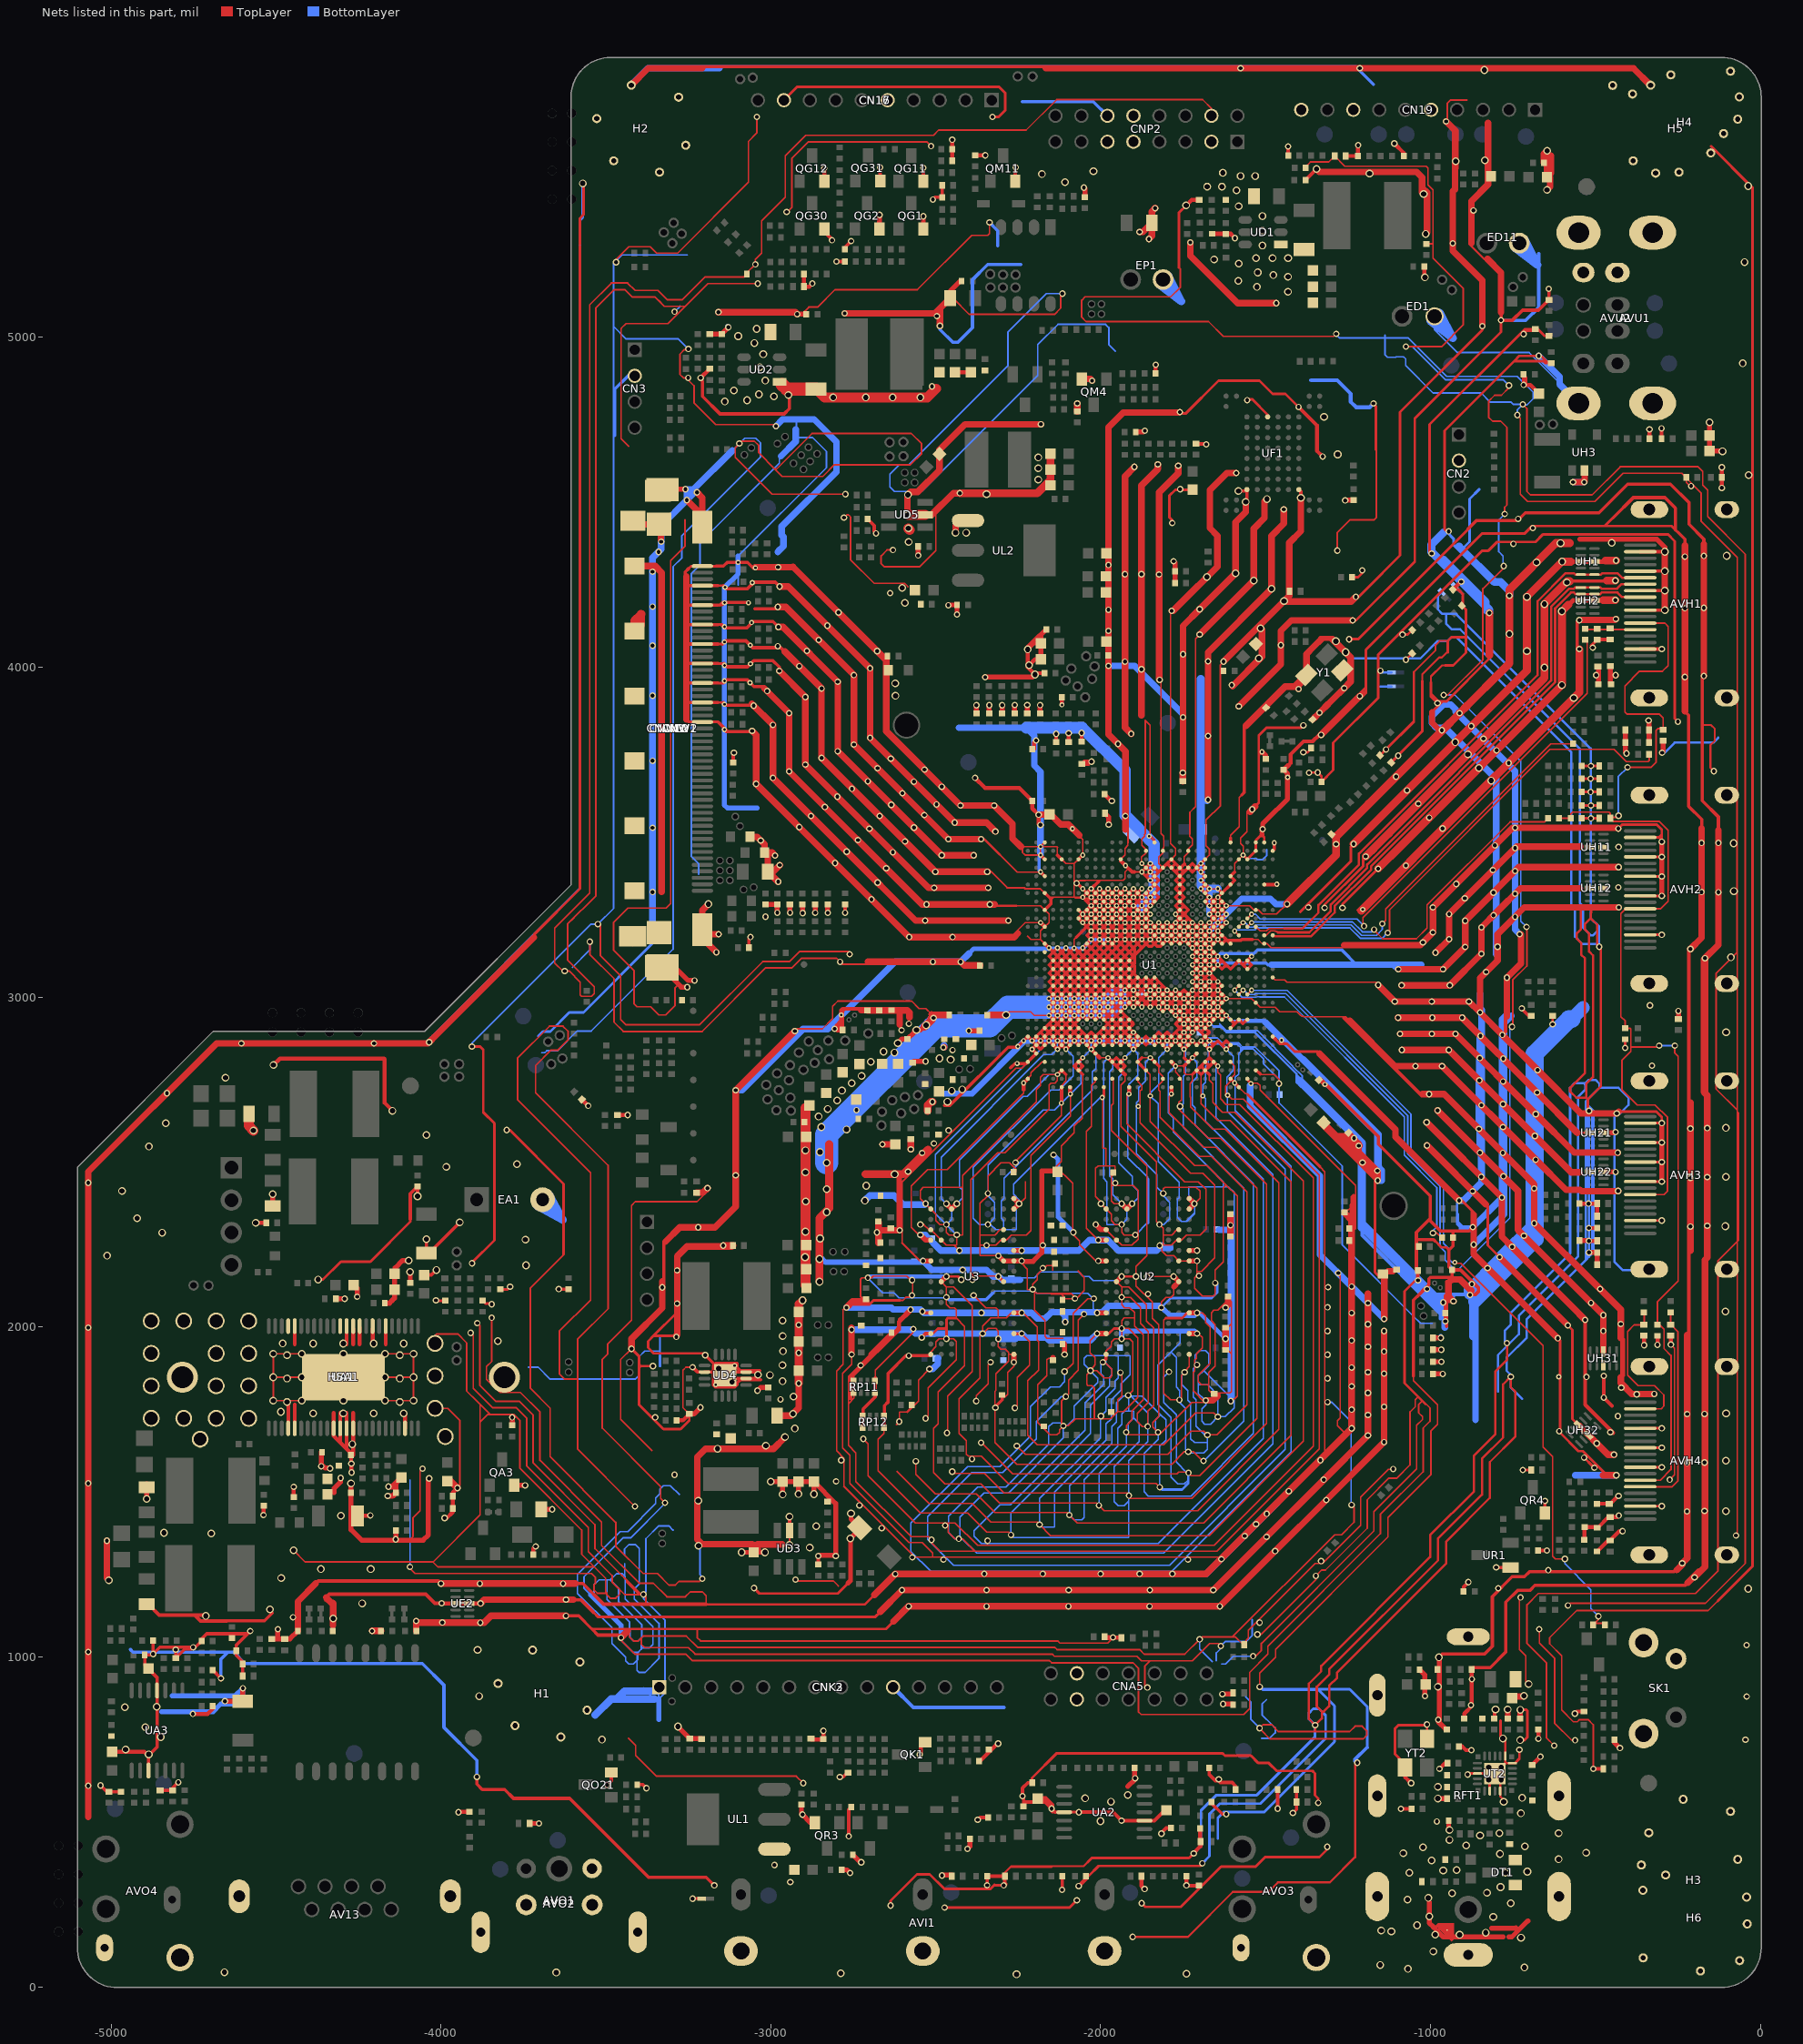
[diagram p0: the nets of this part, all layers, seen from the top]
# Altium PCB MISC86290.PcbDoc (part 21 of 31)
Units mil, origin at the board's own origin, x right, y up, seen from the top; angles counter-clockwise.
Board outline 5104.71 x 5851.49 mil, 2 copper layers (TopLayer, BottomLayer), stack 61.855 mil thick; 1026 components, 667 nets, 4280 pads, 2294 vias.

## Via types
v1: diameter 19.68, hole 11.81, TopLayer to BottomLayer, tented both sides, 1189 vias
v2: diameter 19.68/19.68 (per signal layer), hole 11.81, TopLayer to BottomLayer, tented both sides, 366 vias
v3: diameter 15.75, hole 7.87, TopLayer to BottomLayer, tented both sides, 348 vias
v4: diameter 23.62, hole 15.75, TopLayer to BottomLayer, tented both sides, 309 vias
v5: diameter 15.75/15.75 (per signal layer), hole 7.87, TopLayer to BottomLayer, tented both sides, 59 vias
v6: diameter 24/24 (per signal layer), hole 16, TopLayer to BottomLayer, tented both sides, 23 vias

## Nets (pads, with @x,y where several pads share a name; then routed paths per layer and width w, separated by ;. In a path a pad name is that pad's centre, name@x,y a point inside that pad or via, vN(x,y) a via of type N, cw(c..) or ccw(c..) an arc to the next point about the centre after c; other vN are vias at no path point) (continued)
GND: (continued)
  BottomLayer w15.75: v6@-2849.72,2268.03 -2849.72,2212.2 -2833.98,2196.46 -2542.64,2196.46 v2(-2538.7,2200.39) ; v2(-1936.34,1964.17) -1936.34,1991.73 -1932.4,1987.8 -1759.17,1987.8 -1715.87,1987.8 v2(-1707.99,1979.92) ; v3@-1925.81,2867.72 v3(-1900.91,2867.72) v3@-1867.72,2867.72 ; v3@-1920.59,2867.72 -1910.75,2857.87 ; -1889.09,2857.87 -1879.25,2867.72 v3@-1867.72,2867.72 ; -1857.6,2865.75 -1857.6,2867.72 v3@-1867.72,2867.72 ; v2(-1816.26,2058.66) -1814.29,2058.66 -1790.67,2035.04 -1715.87,2035.04 v2(-1707.99,2042.91)
  BottomLayer w18: -2471.72,2708.03 -2389.72,2708.03 -2230.04,2867.72 -2117.44,2867.72 v3@-1920.59,2867.72
  BottomLayer w19.68: v2(-2770.98,2058.66) -2635.16,2058.66 -2629.25,2052.76 v2(-2576.1,2052.76) -2546.57,2052.76 v2(-2540.67,2046.85) -2536.73,2042.91 v2(-2361.54,2042.91) v2(-2239.49,2042.91) -2209.96,2042.91 -2192.24,2025.2 -2168.62,2025.2 -2148.94,2044.88 -2119.41,2044.88 ; v2(-2755.24,1991.73) -2574.13,1991.73 -2562.32,1979.92 v2(-2357.6,1979.92) v2(-2239.49,1979.92) v2@-2237.66,1978.09 ; v2@-2547.82,2279.13 -2532.07,2279.13 -2484.83,2231.89 ; v2(-2546.57,2279.13) -2530.83,2279.13 ; v2(-2538.7,2200.39) -2511.14,2172.83 v2(-2418.62,2172.83) -2345.79,2172.83 -2326.1,2153.15 v2(-2310.35,2153.15) ; -2483.58,2231.89 v2(-2428.46,2231.89) v2(-2239.49,2231.89) -2066.26,2231.89 -2034.76,2263.39 -1977.68,2263.39 -1946.18,2231.89 -1830.04,2231.89 v2@-1822.25,2239.68 ; v2@-2237.6,1978.03 -2227.68,1968.11 -2164.88,1968.11 -2157.01,1960.24 -2030.83,1960.24 v2(-2011.14,1979.92) ; v2(-2107.6,2015.35) -2107.6,2033.07 -2119.41,2044.88 ; -1897.31,4004.31 v1@-1750.25,3857.25 ; v2(-1816.26,2058.66) -1822.17,2064.57 -1975.71,2064.57 -1995.39,2044.88 -2119.41,2044.88 ; v2@-1814.29,2247.64 v2@-1822.25,2239.68 ; C95.1@-1788.7,2239.59 -1822.17,2239.59 v2@-1822.25,2239.68 ; v1@-1678.07,3594.68 v1(-1674.72,3598.03) ; v3(-1670.59,3200.39) -1572.48,3298.5 -1485.5,3298.5 -1469.21,3282.21 v1(-1434.96,3282.21) ; C85.1@-1640.75,2294.88 -1611.54,2294.88 -1605.63,2288.98 -1605.63,1785.92 v2(-1605.63,1775.2) ; -1501.73,2924.84 -1454.45,2877.56 -1436.82,2859.93
  BottomLayer w20: v4(-3570.25,5467) v4@-3569.83,5466.58 ; H2.3@-3424.48,5764.76 -3373.28,5815.96 -3156.25,5815.96 ; -3358.61,3183 -3358.61,3267 ; -3358.61,3223.74 -3358.61,3267 ; -3332.25,4428.59 -3332.25,4428.75 ; v1@-3224.72,4531.02 -3229.98,4531.02 v1@-3251.75,4509.25 ; -3116.5,4657.2 -3235.31,4538.38 -3254,4538.38 -3254,4511.5 v1@-3251.75,4509.25 ; v1@-3106,2718.25 -3086.97,2718.25 -2902.21,2903 -2827.32,2903 -2623.32,3107 v1(-2509,3107) v1(-2424.51,3107) -2399.15,3132.36 ; v1(-2984.5,4731) -2964.16,4751.34 -2868.71,4751.34 ; -2979,4350 -2976.94,4352.06 -2976.53,4352.06 -2961.97,4366.61 -2961.97,4394.97 -2967,4400 -2967,4426.66 -2801,4592.66 -2801,4683.63 -2868.71,4751.34 ; -2969,4639.91 -2924.41,4684.5 -2924.41,4720.59 ; -2893.66,4751.34 -2868.71,4751.34 ; v6@-2715.97,2383.03 -2700.28,2398.72 ; v6(-2714.72,2383.03) -2699.03,2398.72 -2626.42,2398.72 -2598.42,2370.72 -2533.72,2370.72 v2(-2530.83,2373.62) ; v2(-2519.02,1872.64) -2509.72,1872.64 -2493.72,1888.64 -2493.72,1904.5 C94.1@-2493.11,1905.12 ; v1@-2475,2848 v1@-2475,2854.32 ; -2430,3817 -2225.58,3817 -2201.16,3792.58 -2201.16,3702.01 -2182.4,3683.26 v3(-2182.4,3430.71) ; v2(-2310.35,1964.17) -2257.72,1964.17 -2253.79,1968.11 -2227.68,1968.11 ; v2@-2304.76,2149.21 -2298.54,2142.99 -2290.72,2142.99 ; C93.1@-2270.98,2142.99 -2290.72,2142.99 ; -2243.72,2142.99 -2290.72,2142.99 ; v1(-1976.45,4004.31) -1926,4004.31 ; v1(-1926.45,4017) -1926,4016.55 -1926,4004.31 ; v3(-1900.91,2867.72) -1845.79,2867.72 -1843.82,2865.75 -1857.6,2865.75 ; -1897.31,4004.31 -1926,4004.31 ; -1680.29,1251.34 v2(-1529,1402.63) -1465.58,1466.06 ; v3@-1670.59,3252.21 v3(-1670.59,3328.35) ; v3@-1546.69,2733 -1546.69,2670.24 -1335.17,2458.73 -1335.17,2218.44 v1(-1239.22,2122.5) v1(-1140.72,2024) ; -1481.85,3098.03 -1122,3098.03 ; -1454.45,2877.56 -1425.67,2848.78 -1357.44,2780.56 ; -1384.92,2811.31 -1157.91,2584.3 -1157.91,2476.95 v1(-1161.28,2473.58) ; -1309.76,2732.87 -1357.44,2780.56 ; -1203.17,2307.5 -1203.17,2295.67 -970.5,2063 ; -1182.77,2607.6 -1220.09,2644.91 ; v1@-1161.73,2474.02 -1161.73,2586.55 -1220.09,2644.91 ; v1@-1160.5,2474.36 v1(-1160.5,2444) -1148.5,2444 -1147.5,2445 -1147.5,2475.02 -1159.01,2486.54 -1159.01,2509 ; v1(-1097.72,3084.85) -1110.9,3098.03 -1122,3098.03 ; -1028.32,3098.03 -1122,3098.03 ; -970.5,2081.5 -961.5,2072.5 -957,2072.5 -957,2091.5 -935.76,2091.5 ; -957,1999 -957,2054 ; v1@-913.5,2383.45 -900.55,2383.45 v1(-872.4,2411.6) -844.84,2439.16 v1@-844.84,2453.55 ; -905.29,2298.16 -876.84,2298.16 v1(-872,2303) v1@-783,2392 ; v1(-869.43,2249.54) -783,2336 ; -864,1719 -864,1962 ; -850.23,3010.77 -850.23,2966.38 -844.84,2961 v1@-844.84,2453.55 ; v1(-848.42,2882.42) -850.57,2880.28 v1(-850.57,2815.28) -852.21,2813.63 v1(-852.21,2747.63) -853.27,2746.57 -853.27,2664.57 ; -846.29,2470 v1@-846.29,2456.21 ; v1(-845.86,2671.98) -853.27,2664.57 ; v1(-811,3385) -800.84,3395.16 -800.84,3398 ; v1(-809.31,3317.06) -800.84,3325.53 -800.84,3331 ; v1(-804.9,3460.06) -800.84,3456 -800.84,3419 ; -800.84,3130.84 -800.84,3331 ; v1@-783,2885.54 -783,2854.5 ; -772.84,2943 -783,2932.84 -783,2854.5 ; -754.63,2943.5 -777.84,2920.29 -777.84,2394.66 -777.18,2394 -777.18,2341.82 -783,2336 ; -747,2181.13 -792.5,2135.63 ; v1(-730,3191) -743.84,3204.84 -743.84,3685.26 -923.79,3865.21 -923.79,3871.92 -938.71,3886.84 -960.29,3886.84 -995.84,3851.29 -995.84,3830.71 -981.29,3816.16 -960.71,3816.16 -958.03,3818.84 -800.84,3661.65 -800.84,3419 ; -677.5,2331.26 -692.18,2316.57 -792.5,2216.26 -792.5,2199.5 -792.5,2161.5 ; v1(-672,4944) -609,4881 -609,4862 -609,4858.21 AVU2.9@-551.16,4800.38 ; v1(-568,4561.43) v1(-534,4561.43) ; -561,1550.66 v2(-437,1550.66) ; -3358.61,3267 -3358.61,4331.67 -3332.41,4357.88 v1(-3332.41,4380.97) -3332.41,4428.59 -3332.25,4428.75 ; -3332.25,4428.75 v1@-3251.75,4509.25 ; -1357.44,2780.56 -1355.73,2780.56 -1220.09,2644.91 ; -864,1962 -864,2064.13 -792.5,2135.63 ; -864,1962 -873,1971 -873,2081 -792.5,2161.5 ; -853.27,2664.57 v1(-853.27,2600.57) -850.42,2597.72 v1(-850.42,2528.42) -846.29,2524.3 v1@-846.29,2456.21 ; v1@-846.29,2456.21 v1(-846.29,2455) v1@-844.84,2453.55 ; -800.84,3331 -800.84,3398 ; -800.84,3398 -800.84,3419 ; -792.5,2135.63 -792.5,2149.77 -792.5,2161.5 ; -783,2336 v1@-783,2392 ; v1@-783,2392 -783,2854.5
  BottomLayer w23: -3532.25,824 -3484.25,872 -3468,872 ; -3353,872 -3468,872 ; CNK2.1@-3339.87,900.87 -3344.55,896.19 -3377.19,896.19 -3443.81,896.19 -3468,872
  BottomLayer w24: v6@-2524,2923 v1@-2512.97,2934.03 ; v1@-998.61,4351 v1@-997.24,4349.63 ; -960.38,4408.72 -997.24,4371.87 v1@-997.24,4349.63 ; -913.59,4365.41 -905.09,4356.91 -806.64,4258.46 -787.88,4258.46 -761,4231.58 v1(-761,4217) ; v1@-997.24,4349.63 -973.44,4325.83 ; v1@-997.24,4349.63 -996.91,4349.3 -973.44,4325.83 ; -973.44,4325.83 -960.28,4325.83 -832.84,4198.4 -832.84,4185.24 ; -973.44,4325.83 -962.8,4315.2 ; -973.44,4325.83 -962.8,4315.2 ; -962.8,4315.2 -832.84,4185.24 ; -832.84,4185.24 -822,4174.39 v1(-822,4165) -832.84,4175.84 -832.84,4185.24
  BottomLayer w25: -1696.18,3963.97 v3(-1696.18,3405.12) v3(-1696.18,3379.53) v3(-1696.18,3353.94) -1696.18,3336.49 -1688.51,3328.82 -1645.47,3328.82 v3(-1645,3328.35) ; -1396.91,2745.73 -1208.37,2557.2 -1208.37,2300.87
  BottomLayer w35: -2225.58,3817 -2056,3817 -1926,3687 -1926,3587 ; v1@-1926,3554.11 -1926,3587 ; v3(-1875.32,3277.17) -1838.22,3314.26 -1838.22,3463.44 -1926,3551.22 -1926,3587
  BottomLayer w40: v1@-879.86,2102.14 -879.86,2112.14 -792.5,2199.5 -692.18,2299.82 ; -865.16,2077.12 -792.5,2149.77 -677.5,2264.77 v1@-677.5,2314.5 ; -537.86,2968.14 -572.5,2933.5 -677.5,2828.5 ; -692.18,2299.82 -692.18,2316.57 -692.18,2813.82 -677.5,2828.5 ; -692.18,2299.82 v1@-677.5,2314.5 ; v1@-677.5,2314.5 -677.5,2331.26 -677.5,2828.5
  BottomLayer w54: -684.5,2797.38 -684.5,2828.67 -579.67,2933.5 -572.5,2933.5
  BottomLayer w70: v6(-2830.97,2498.03) -2830.97,2582.6 -2500.57,2913 -2337.26,2913 -2281.22,2969.03 -1976.72,2969.03 v3@-1950.17,2995.59
  other v1: -2941,317 -980.96,501.01 -5069.17,609 -2311,737 -45.5,748.5 -41.5,880 -5069.17,1015 -42,1035.5 -1963,1059 -4448.5,1120 -795,1208 -222.5,1441 -169.5,1442.5 -5069.17,1526 -3292,1552 -503.55,1573.5 -4363.02,1577.8 -222.5,1588 -169.5,1589 -610,1684 -3350.5,1726 -1189.72,1733.5 -222.16,1736 -169.5,1736.5 -1239.22,1749.5 -1140.72,1758 -2970.5,1780.5 -1189.72,1800 -422,1816 -1239.22,1820 -1140.72,1858.5 -1189.72,1863 -1239.22,1877 -1140.72,1926 -1189.72,1940 -1239.22,1959 -3286.5,1970 -1189.72,2008.5 -423.5,2009 -1239.22,2042.5 -3284,2071 -961.5,2074.5 -3329,2120 -1311,2121 -875,2130 -3284,2172 -3220,2302 -212.16,2304.5 -521,2374 -5069.17,2437 -212.16,2451.5 -778.96,2456.74 -2541.5,2527.5 -780.87,2527.94 -2505.5,2556.5 -212.16,2601.5 -780.19,2606.07 -2740.5,2657.5 -780.48,2675.67 -4831,2708.9 -779.97,2744.46 -1046.07,2790.85 -329,2792.5 -779.59,2813.5 -2449,2839.5 -2477,2847.5 -4605,2859.89 -4203,2859.89 -996,2888.85 -2603.5,2899.5 -2806.43,2903.66 -630,2918 -2581.5,2919.5 -2506.5,2937 -995,2937.85 -335,2975 -996.5,2986.85 -3253.5,3030 -831.57,3076.43 -2761,3130 -2532,3232.11 -743.84,3243.5 -3016,3244 -2528,3281.11 -2694.91,3296.55 -896.01,3299.88 -743.64,3313.65 -3358.61,3318.5 -127.41,3318 -2505,3331.11 -922,3343.18 -2676.47,3347.4 -2977.5,3350 -743.84,3382.5 -2650.17,3390.4 -2629.87,3439.39 -743.84,3452 -430,3455 -2593.25,3472.08 -2735.77,3476 -2701,3510.53 -963.56,3511.29 -3358.5,3513.5 -743.84,3513.5 -2565.88,3513.99 -2913.78,3515.42 -514,3542 -1003.96,3544.19 -2878.45,3549.38 -2670.18,3549 -1925.13,3549 -2534.47,3551.88 -2836.23,3576.46 -2634.88,3583 -2497.46,3584.17 -1037,3586.5 -2798.44,3607.97 -2601,3618.41 -515,3622 -1071.18,3626.87 -2754.33,3631.63 -2481.87,3637.88 -2566.29,3653 -2706,3654.5 -1104.62,3668.39 -2534,3690 -2676.62,3694.03 -763.36,3709.84 -3358.61,3716.5 -2636.27,3722.98 -800.03,3748.12 -1947.63,3767.63 -839.68,3783.43 -1674.72,3792 -966,3809 -876.66,3821.4 -1750.25,3848.5 -1336.49,3862.35 -3052,3883.75 -3358.61,3914 -3011,3928 -1821.25,3962 -2350,3970 -2913.65,4003.2 -1674.72,4018 -1750.25,4039.5 -2677.52,4049 -2891,4050 -2979,4064 -3358.61,4065.5 -2854.67,4082.81 -1976.78,4110.3 -2828.41,4126.16 -2794.89,4166.36 -1976.78,4174.3 -3358.61,4184 -2638.5,4225 -1823,4281.5 -1926.45,4282 -1876.45,4282 -3358.5,4289.5 -2978,4303.5 -1976.45,4310 -3340.5,4349.5 -3255,4507 -1759,4540 -3095.5,4678.5 -2511.46,4851.46 -2496.77,5064.66 -933,5285 -870,5385 -2509,5418 -2257.5,5515.5 -1576,5815.96 -1214.5,5815.96
  other v2: -671,1084 -3881,1103.5 -3996,1104 -2346,1153.11 -1852,1153.11 -3621,1173.16 -2346,1202.11 -1851,1202.11 -3630,1222.16 -2352.68,1251.57 -2175.51,1251.57 -2000.32,1251.57 -1882.2,1251.57 -1782.8,1251.57 -2476.69,1294.88 -1735.55,1294.88 -1634.17,1295.87 -2571.18,1301.77 -2342.83,1351.97 -1563.31,1366.73 -2663.7,1390.35 -2471.77,1398.23 -429.33,1428.13 -1496.38,1433.66 -299,1456.64 -2731.61,1459.25 -2802,1532 -299,1574.75 -2786.73,1596.06 -1333.98,1596.06 -2390.08,1600 -299,1633.8 -455,1681 -299,1692.86 -432,1730 -375,1796 -1312.32,1844.09 -2727.68,1883.46 -1312.32,1915.94 -1312.32,1987.8 -1312.32,2059.65 -1856.61,2100 -2389.09,2143.31 -1702.09,2155.12 -2175.51,2178.74 -2175.51,2247.64 -1821,2247 -2678.46,2287.01 -2609.57,2292.91 -1606.61,2308.66 -299,2322.78 -1956.02,2436.61 -299,2440.89 -2583.98,2471.06 -299,2499.94 -2461.21,2596.06 -299,3188.92 -299,3307.03 -431,3333 -299,3366.09 -299,3425.14 -1603,3946
  other v3: -3167,1825 -611.5,1849 -3110,1883 -2182.4,2867.72 -1452,2869.29 -2131.22,2944.49 -2105.63,2944.49 -2080.04,2944.49 -2054.45,2944.49 -2028.86,2944.49 -2003.27,2944.49 -2131.22,2970.08 -2105.63,2970.08 -2080.04,2970.08 -2054.45,2970.08 -2028.86,2970.08 -2003.27,2970.08 -1977.68,2970.08 -1798.54,2970.08 -1772.95,2970.08 -2131.22,2995.67 -2105.63,2995.67 -2080.04,2995.67 -2054.45,2995.67 -2028.86,2995.67 -2003.27,2995.67 -1977.68,2995.67 -1952.09,2995.67 -1926.5,2995.67 -1900.91,2995.67 -1849.72,2995.67 -1824.13,2995.67 -1798.54,2995.67 -1619.41,2995.67 -1926.5,3021.26 -1900.91,3021.26 -1849.72,3021.26 -1696.18,3021.26 -1696.18,3046.85 -1696.18,3072.44 -1670.59,3072.44 -1696.18,3098.03 -1670.59,3098.03 -1696.18,3123.62 -1670.59,3123.62 -1619.41,3123.62 -2156.81,3149.21 -2054.45,3149.21 -1696.18,3149.21 -2003.27,3174.8 -1952.09,3174.8 -1926.5,3174.8 -1900.91,3174.8 -1875.32,3174.8 -1798.54,3174.8 -1772.95,3174.8 -1747.36,3174.8 -1670.59,3174.8 -2028.86,3200.39 -2003.27,3200.39 -1977.68,3200.39 -1952.09,3200.39 -1926.5,3200.39 -1900.91,3200.39 -1875.32,3200.39 -1849.72,3200.39 -1824.13,3200.39 -1798.54,3200.39 -1772.95,3200.39 -1747.36,3200.39 -2028.86,3225.98 -2003.27,3225.98 -1977.68,3225.98 -1952.09,3225.98 -1926.5,3225.98 -1900.91,3225.98 -1875.32,3225.98 -2054.45,3251.57 -2028.86,3251.57 -2003.27,3251.57 -1977.68,3251.57 -1952.09,3251.57 -1926.5,3251.57 -1900.91,3251.57 -1875.32,3251.57 -1205.78,3265.86 -2028.86,3277.17 -2003.27,3277.17 -1977.68,3277.17 -1952.09,3277.17 -1926.5,3277.17 -1900.91,3277.17 -2028.86,3302.76 -2003.27,3302.76 -1977.68,3302.76 -1952.09,3302.76 -1926.5,3302.76 -1900.91,3302.76 -1849.72,3379.53 -1875.32,3405.12 -2085.8,3510.43
  other v4: -2255,37.5 -1740,39.5 -2788,40.5 -3650.5,43 -4656,44 -1068.34,54.06 -715.34,58.06 -1152.34,66.06 -991.77,106.7 -725.84,148.7 -912.03,157.38 -986,158 -833,164 -1118.82,167.61 -1149.47,170.45 -1041.24,186.1 -810,212 -756.7,253.3 -1070,264 -1007,269 -935,283 -829,285 -787.86,302.07 -1064.7,345.3 -772.86,345.07 -706.5,348.81 -961.7,352.3 -920.7,353.3 -996.7,382.3 -611.63,386.36 -789.53,402.65 -1082.82,404.61 -528.5,406 -1022.82,422.61 -714.3,425.41 -891.7,428.3 -942.53,445.15 -850.03,458.15 -791.03,465.5 -611.63,465.21 -2001,502 -726.03,525.65 -1969,561 -978.03,570.65 -2047,571 -722.03,572.38 -1918,581 -978.03,605.65 -823.59,627.66 -786.19,627.66 -823.59,665.07 -786.19,665.07 -4886,704.5 -4956,719.5 -3512,749 -4849.5,757 -4896.5,786.5 -803.03,840.66 -766.03,840.65 -4958.5,847.5 -4862,848.5 -3884,881 -978,909 -3889,1021 -4326.5,1116 -4518.5,1144 -4239,1162.29 -37.5,1206.5 -4484.5,1239 -4364,1266 -4213,1266 -2882.22,1331.72 -3219,1337 -4696,1374 -4839.6,1376.13 -2862.54,1395.78 -4303.5,1427.5 -105,1442 -3220,1473 -4892,1479 -105,1595 -3162,1631 -3015,1640 -4268.68,1644.87 -2927.5,1692 -2933,1737 -4387.55,1737.87 -4295.93,1737.87 -4204.3,1737.87 -4112.68,1737.87 -104,1738 -4485,1743 -4508.35,1776.88 -4421.73,1776.88 -4295.75,1776.88 -4169.77,1776.88 -4083.15,1776.88 -2931,1789.5 -3117.54,1833.29 -2964.5,1835.5 -4508.35,1847.75 -4421.73,1847.75 -4295.75,1847.75 -4169.77,1847.75 -4083.15,1847.75 -3002.5,1854.5 -3158.48,1874.08 -2965,1884 -4508.35,1918.61 -4421.73,1918.61 -4295.75,1918.61 -4169.77,1918.61 -4083.15,1918.61 -2963,1926.5 -4480,1950 -4387.55,1949.75 -4295.93,1949.75 -4204.3,1949.75 -4112.68,1949.75 -3828,1957 -2964,1972.5 -2964.5,2019.5 -106,2047 -3742,2187 -5012,2216 -3744,2265 -4845,2286 -2895,2289 -106.5,2305.5 -4921,2330 -2894,2381 -4967,2412 -105,2455.5 -2894.97,2468.5 -3984,2485.4 -3770,2494 -2894.97,2535.5 -4885,2547 -4044,2582 -2770.5,2599 -105,2603.5 -4834,2618 -2855,2638 -2827.5,2661 -2799,2686.5 -2784.5,2716.5 -2754.5,2739 -4653,2756 -2725,2761 -2697,2804 -2625.5,2832 -2658.5,2835 -104,2893.7 -89.5,3120.5 -80.5,3321.5 -81,3466.5 -816.58,3656.62 -853.77,3694.38 -886.92,3736.18 -925.32,3772.73 -565.84,3907.36 -2622,3913.5 -2623,3951.5 -655,3999 -1521,4027 -1257.72,4045.72 -708,4049 -1287,4079 -761,4101 -1515.08,4118.08 -2593.5,4195 -1444.34,4200.66 -2601.5,4240.5 -586.71,4257.48 -1678,4274 -678.82,4317.72 -102.5,4338 -606,4376.36 -450.53,4377.39 -2582,4380 -2440,4408 -2408,4408 -2346,4524.78 -2189,4569 -36,4583 -2189,4603 -2189,4636 -1281.5,4645.5 -115,4655 -1323,4759.5 -3139.5,4805.5 -3072,4809.5 -2811,4818 -2712,4818 -2631,4818 -2546.5,4818 -2990.5,4821.5 -2947,4825 -3036.5,4827.5 -3112,4839 -3017,4869 -3034,4910 -54,4921.5 -3023,4949 -3050,4983 -3099,5004 -3043,5026 -1432,5138 -1526,5153 -1582.5,5171.5 -1017,5182 -1432,5184 -1477,5189 -1524,5197 -1581.77,5224.18 -48,5228.5 -1656.5,5236.5 -1528.77,5240.18 -1479,5240.18 -1431.81,5240.18 -1582,5397.66 -1588,5446 -37,5459 -2108,5471 -2178,5495 -1185,5497 -2022,5504 -924,5534 -835.46,5537 -837,5810.5
  other v5: -1886.14,2668.9
  other v6: -2852.5,2137 -2852.5,2206 -2896,2212 -2850.97,2268.03 -2830.97,2348.03 -2830.97,2418.03 -2710.97,2428.03 -2624.72,2463.03 -2851,2530 -2846.97,2606.03 -2464.5,2683 -2451.5,2716 -2419.58,2720.17 -2455,2810.5 -2488.5,2814.5 -2558.5,2900.5
GPIO2_PM/RST_INHN: R153.2 RR4.1 U1.M4 | length 2515.7
  TopLayer w3.94: U1.M4@-1555.43,3008.46 v3(-1542.64,3021.26)
  TopLayer w5: v3(-926.47,2195.72) -926.47,2194.37 -927.86,2192.98 -908.52,2192.98 -658.88,1943.35 -658.88,1635.81 -629.84,1606.77 -629.84,1304.84 -622,1297 v1(-593,1297) ; R153.2@-507,1097 R153.2@-502,1102 ; v1(-491,1123) -491,1113 R153.2@-502,1102 ; RR4.1@-471.73,1097 -471.73,1102 R153.2@-502,1102
  BottomLayer w5: v3@-1541.91,3020.53 -1434.61,3020.53 -1059.5,2645.43 -1059.5,2529.15 -961,2430.65 -961,2253.5 -945.66,2238.16 -945.66,2207.16 -934.21,2195.72 v3(-926.47,2195.72) ; v1(-593,1297) -593,1282.5 -514,1203.5 -514,1146 v1(-491,1123)
GPIO9_PM: R151.1 U1.N5 | length 1114.4
  TopLayer w3.94: v3(-1593.82,3021.26) U1.N5@-1581.02,3034.06
  TopLayer w5: v1(-992.5,2285) -981.59,2285 -967.89,2271.3 R151.1@-965.5,2271.3
  BottomLayer w3.94: v3(-1593.82,3021.26) -1572.17,2999.61 -1527.22,2999.61 ; -1526.3,3000.53 -1517.22,3000.53
  BottomLayer w5: -1517.22,3000.53 -1442.89,3000.53 -1079.5,2637.14 -1079.5,2520.87 -981,2422.37 -981,2303.5 v1@-992.5,2292
GPIO10_PM/HOST_WAKE_WIFI: DW1.K R152.2 RU17.2 U1.M5 | length 5774.8
  TopLayer w3.94: U1.M5@-1581.02,3008.46 v3(-1568.23,3021.26)
  TopLayer w5: RU17.2@-1378.27,5514 -1378.27,5517.73 -1364,5532 -1308.73,5532 DW1.K@-1290.73,5550 -1259.73,5519 -1013,5519 -1008,5514 -1008,5462.86 -992.75,5447.61 -992.75,5240.73 -901.09,5149.07 -901.09,5037.81 -966.9,4972 v1(-1075,4972) ; R152.2@-1013,5283.73 -994.48,5283.73 ; v1(-960,3916) -948.23,3916 -841.5,4022.73 -841.5,4238.36 -778,4301.86 v1(-778,4307) ; v1(-775.11,4464.84) -775.11,4485.42 -768.66,4491.87 -768.66,4727.65 -787.01,4746 -812.14,4746 -824,4757.86 -824,4806.6 -805.84,4824.76 -785.07,4824.76 -762.37,4847.46 v1(-762.37,4854.16) ; v1@-751,2912 -751,3051.64 -708.34,3094.3 -708.34,3212.34 v1(-709,3213)
  BottomLayer w3.94: v3@-1566.4,3021.26 -1552.48,3007.48 -1532.8,3007.48 -1529.83,3010.44 -1525.24,3010.44
  BottomLayer w5: -1525.15,3010.53 -1438.75,3010.53 -1069.5,2641.28 -1069.5,2525.01 -971,2426.51 -971,2242.72 -955.66,2227.37 -955.66,2203.02 -929.29,2176.66 -913.42,2176.66 -759.68,2330.39 -759.68,2903.32 v1(-753,2910) ; v1(-1075,4972) -1055.14,4972 -955.14,4872 -780.21,4872 v1(-762.37,4854.16) ; v1(-960,3916) -927,3916 -726.34,3715.34 -726.34,3230.34 v1(-709,3213) ; v1(-778,4307) -780,4309 -780.32,4309 -780.32,4337.53 -793.34,4350.55 -793.34,4446.61 v1(-775.11,4464.84)
GST_VST: U1.U28
HDMI-ARC_IC: CH7.2 U1.AA4 | length 1535.3
  TopLayer w5: U1.AA4@-1555.43,3238.78 v3(-1542.64,3251.57) ; v1(-1201.37,3215.1) -1205,3211.47 -1205,3240.62 -525.34,3920.28 -525.34,4077.61 CH7.2@-531,4083.27
  BottomLayer w5: v3(-1542.64,3251.57) -1531.07,3251.57 -1516.27,3236.77 -1223.04,3236.77 v1(-1201.37,3215.1)
HDMI-CEC_IC: RH17.2 U1.Y4 | length 1139
  TopLayer w3.94: U1.Y4@-1555.43,3213.19 v3(-1542.64,3225.98)
  TopLayer w5: v1(-1171,3205) -1172,3204 -1145,3177 -1043,3177 -1010.5,3209.5 -1010.5,3279.43 -758.93,3531 -654.73,3531 RH17.2@-643.73,3542
  BottomLayer w5: v3(-1542.64,3225.98) -1540.76,3227.87 -1237.11,3227.87 -1207,3197.76 -1178.24,3197.76 v1(-1171,3205)
HDMI_ARC: AVH1.14 CH6.1 CH7.1 DH5.K | length 168.7
  TopLayer w5: CH7.1@-532.25,4116.73 CH7.1@-529.71,4116.73 ; CH7.1@-529.69,4114.18 AVH1.14@-364.47,4114.18 ; CH7.1@-528.46,4116.73 CH7.1@-527.8,4116.07
HDMI_CEC: AVH1.13 AVH2.13 AVH3.13 AVH4.13 CH15.2 CH16.2 CH17.2 CH18.2 DH15.K RH17.1 | length 4370.8
  TopLayer w5: RH17.1@-610.26,3541.99 CH17.2@-574.73,3541.99 -574.73,3555.27 -569,3561 -459.17,3561 -455.27,3557.09 DH15.K@-455.27,3542 ; v2(-430,3550) -435,3545 -452.27,3545 DH15.K@-455.27,3542 ; v2(-402.85,3696.66) -332.34,3696.66 -316,3713 -316,3809 -311.32,3813.68 -304.84,3813.68 ; AVH1.13@-365.72,4133.86 -289.86,4133.86 -280,4124 -280,4005 -297,3988 -366.1,3988 -411,3943.1 -411,3864.41 -404.86,3858.27 -307.27,3858.27 -295,3846 CH16.2@-295,3810.73 ; AVH4.13@-364.47,1535.43 -303.57,1535.43 -271,1568 -271,1913.5 -292,1934.5 -292,1993 -305.73,2006.73 CH15.2@-312,2006.73 -312,2077.5 -249.66,2139.84 -249.66,2820.8 -259.5,2830.64 v2(-259.5,2853) ; AVH3.13@-364.47,2401.58 -292.08,2401.58 -281.66,2412 -281.66,2635.31 -319.35,2673 -373,2673 -420,2720 -420,2808 -392.66,2835.34 -392.66,2849 ; v2(-307,2853) -311,2849 -392.66,2849 ; DH15.K@-455.27,3542 -446.27,3533 -307.18,3533 -280,3505.82 -280,3291 -303.28,3267.72 AVH2.13@-364.47,3267.72 -409.22,3267.72 -423,3253.94 -423,2941 -410,2928 CH18.2@-410,2905.73 -395.73,2905.73 -392.66,2902.66 -392.66,2849
  BottomLayer w5: v2@-431,3550 -431,3668.51 v2(-402.85,3696.66) ; v2(-307,2853) v2(-259.5,2853)
HDMI_UART_RX: AVH4.2 DH35.K RH38.1 | length 472.2
  TopLayer w5: AVH4.2@-364.47,1751.97 -301.03,1751.97 -293,1760 -293,1794 -321,1822 -371,1822 -402.76,1853.76 -402.76,1986.74 -383.27,2006.23 -352.5,2006.23 RH38.1@-352.5,2043.77
HDMI_UART_TX: AVH4.14 DH36.K RH37.1 | length 641.8
  TopLayer w5: AVH4.14@-364.47,1515.75 -267.75,1515.75 -250.5,1533 -250.5,1986.23 -272,2007.73 RH37.1@-272,2044.77
HDMIA-DETECT: RH4.1 U1.Y5 | length 1316.1
  TopLayer w3.94: U1.Y5@-1581.02,3213.19 v3(-1568.23,3225.98)
  TopLayer w5: v1(-1146.46,3222.72) -1136,3233.18 -1136,3267.19 -635.19,3768 RH4.1@-567.73,3768
  BottomLayer w3.94: v3(-1568.23,3225.98) -1562.07,3225.98 -1548.33,3212.24 -1536.95,3212.24 -1530.22,3218.97 -1529.47,3218.97
  BottomLayer w5: -1529.47,3218.97 -1240.79,3218.97 -1209.35,3187.52 -1163.95,3187.52 -1146.46,3205.02 v1(-1146.46,3222.72) v1@-1151.72,3222.72
HDMIA-HOTPLUG: RH1.1 U1.W5 | length 1609.3
  TopLayer w3.94: v3(-1593.82,3200.39) U1.W5@-1581.02,3187.6
  TopLayer w5: v1(-1130,3195) -1126,3195 -1124.4,3196.6 -1124.4,3264.65 -638.05,3751 -444,3751 -407,3714 -341,3714 -337.27,3717.73 RH1.1@-337.27,3736 RH1.1@-337.27,3741
  BottomLayer w3.94: v3(-1593.82,3200.39) -1589.81,3204.4 -1531.44,3204.4 -1525.78,3210.07
  BottomLayer w5: -1525.78,3210.07 -1244.48,3210.07 -1212.44,3178.03 -1146.97,3178.03 v1(-1130,3195)
HDMIA-RX0N: AVH1.9 U1.W1 UH2.2 UH2.7 | length 1703.9
  TopLayer w7: U1.W1@-1478.66,3187.6 -1475.35,3184.29 -1362.74,3184.29 -1290.85,3256.18 -1290.85,3275.71 -1180.06,3386.5 -1180.06,3397.09 -622.5,3954.64 -622.5,4178.17 -574.26,4226.4 -565.25,4226.4 -560.9,4222.05 UH2.2@-544.19,4222.05 -485.77,4222.05 -481.42,4226.4 -433.16,4226.4 -419.36,4212.6 AVH1.9@-365.72,4212.6
HDMIA-RX0P: AVH1.7 U1.W2 UH2.1 UH2.8 | length 1751.7
  TopLayer w3.94: U1.W2@-1504.25,3187.6 -1498.35,3187.6 -1485.55,3200.39 -1472.84,3200.39 ; -1463.55,3197.42 ccw(c-1470.73,3190.24) -1470.73,3200.39 -1472.84,3200.39 ; -1462.75,3195.2 cw(c-1462.75,3197.66) -1464.49,3195.92 -1466.22,3197.65 ccw(c-1466.34,3197.53) -1466.28,3197.69 ; -1472.84,3200.39 cw(c-1472.84,3191.08) -1466.28,3197.69 ; -1472.84,3200.39 cw(c-1472.84,3191.2) -1466.34,3197.7 cw(c-1466.34,3197.53) -1466.28,3197.69
  TopLayer w7: -1463,3196.29 -1367.71,3196.29 -1302.85,3261.15 -1302.85,3280.68 -1192.06,3391.47 -1192.06,3402.06 -634.5,3959.61 -634.5,4183.14 -579.23,4238.4 -565.25,4238.4 -561.91,4241.74 UH2.1@-544.19,4241.74 UH2.8@-503.25,4241.74 -484.99,4241.74 -481.65,4238.4 -434.53,4238.4 -420.97,4251.97 AVH1.7@-365.72,4251.97
HDMIA-RX1N: AVH1.6 U1.Y3 UH1.4 UH1.5 | length 1808.1
  TopLayer w3.94: U1.Y3@-1529.84,3213.19 -1517.05,3200.39 -1497.36,3200.39 -1489.49,3208.27 -1445.94,3208.27 ; -1441.84,3208.27 -1445.94,3208.27 ; -1445.94,3208.27 cw(c-1442.72,3205.05) -1442.72,3209.6 ccw(c-1442.72,3205.05) -1445.94,3208.27 ; -1445.94,3208.27 ccw(c-1441.91,3212.29) -1441.91,3206.6 cw(c-1441.91,3212.29) -1445.94,3208.27
  TopLayer w7: -1441.84,3208.11 -1387.97,3208.11 ; -1387.97,3208.29 -1339.96,3256.3 -1339.96,3278.93 -1217.06,3401.83 -1217.06,3435.04 -675.5,3976.59 -675.5,4200.12 -590.16,4285.46 -565.25,4285.46 -560.73,4280.94 UH1.4@-544.19,4280.94 UH1.5@-503.25,4280.94 -483.3,4280.94 -478.79,4285.46 -433.16,4285.46 -419.36,4271.66 AVH1.6@-365.72,4271.66